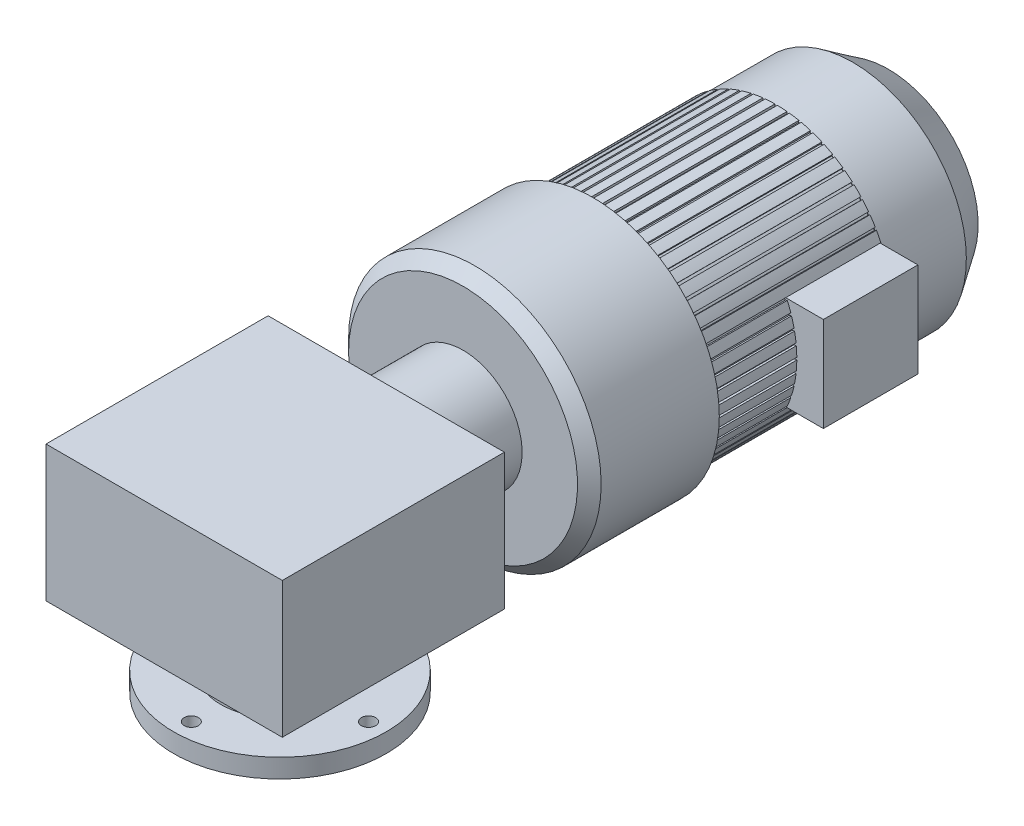
SolidWorks part; units mm, degrees
ref_plane "Front Plane" through (0, 0, 0) normal (0, 0, 1) x (1, 0, 0)
ref_plane "Top Plane" through (0, 0, 0) normal (0, 1, 0) x (1, 0, 0)
ref_plane "Right Plane" through (0, 0, 0) normal (1, 0, 0) x (0, 0, -1)
sketch "Sketch1" plane through (0, 0, 0) normal (0, 0, 1) x (1, 0, 0)
  circle A0 centre (0, 0) radius 16
  dimension "D1" = 32
extrude "Boss-Extrude1" add sketch "Sketch1" along normal blind 55 contours A0
sketch "Sketch2" plane through (0, 0, 0) normal (0, 0, -1) x (-1, 0, 0)
  circle A0 centre (0, 0) radius 22.5
  dimension "D1" = 45
extrude "Boss-Extrude2" add sketch "Sketch2" along normal blind 5
sketch "Sketch3" plane through (0, 0, -5) normal (0, 0, -1) x (-1, 0, 0)
  circle A0 centre (0, 0) radius 25
  dimension "D1" = 50
extrude "Boss-Extrude3" add sketch "Sketch3" along normal blind 5
sketch "Sketch4" plane through (0, 0, -10) normal (0, 0, -1) x (-1, 0, 0)
  circle A0 centre (0, -30.4) radius 50
  dimension "D2" = 100
  dimension "D1" = 30.4
extrude "Boss-Extrude4" add sketch "Sketch4" along normal blind 65
sketch "Sketch5" plane through (0, 0, -75) normal (0, 0, -1) x (-1, 0, 0)
  circle A0 centre (0, -30.4) radius 106.9
  dimension "D1" = 213.8
extrude "Boss-Extrude5" add sketch "Sketch5" along normal blind 110
sketch "Sketch6" plane through (0, 0, -185) normal (0, 0, -1) x (-1, 0, 0)
  circle A0 centre (0, -30.4) radius 97.5
  dimension "D1" = 195
extrude "Boss-Extrude6" add sketch "Sketch6" along normal blind 155
sketch "Sketch7" plane through (0, 0, -340) normal (0, 0, -1) x (-1, 0, 0)
  line L1 (-1, 69.1) -> (1, 69.1)
  line L2 (-1, 69.1) -> (-1, 65.1)
  line L3 (-1, 65.1) -> (1, 65.1)
  line L4 (1, 69.1) -> (1, 65.1)
  line L5 (-1, 69.1) -> (1, 65.1) construction
  line L6 (-1, 65.1) -> (1, 69.1) construction
  circle A0 centre (0, -30.4) radius 97.5 construction
  circle A1 centre (0, -30.4) radius 97.5 construction
  point P0 (0, 67.1)
  dimension "D1" = 2
  dimension "D2" = 2
extrude "Cut-Extrude1" cut sketch "Sketch7" against normal up to surface (155 mm away) up to face at (-97.5, -30.4, -185)
pattern_circular "CirPattern1" count 60 over 360 about axis through (0, -30.4, 0) along (0, 0, 1) of "Cut-Extrude1"
sketch "Sketch8" plane through (0, 0, -340) normal (0, 0, -1) x (-1, 0, 0)
  circle A0 centre (0, -30.4) radius 96
  dimension "D1" = 192
extrude "Boss-Extrude7" add sketch "Sketch8" along normal blind 95
chamfer "Chamfer1" distance 30 distance2 20 1 edges at (-96, -30.4, -435)
sketch "Sketch13" plane through (0, 0, 0) normal (1, 0, 0) x (0, 0, -1)
  line L0 (405, -30.4) -> (75, -30.4) construction
  line L1 (405, -126.4) -> (405, 65.6) construction
  line L2 (75, 76.5) -> (75, -137.3) construction
  line L4 (340, 9.6) -> (260, 9.6)
  line L5 (340, 9.6) -> (340, -70.4)
  line L6 (340, -70.4) -> (260, -70.4)
  line L7 (260, 9.6) -> (260, -70.4)
  line L8 (340, 9.6) -> (260, -70.4) construction
  line L9 (340, -70.4) -> (260, 9.6) construction
  point P6 (300, -30.4)
  dimension "D1" = 80
  dimension "D2" = 80
  dimension "D3" = 105
sketch "Sketch14" plane through (0, 0, -10) normal (0, 0, 1) x (1, 0, 0)
  line L1 (-100, -87.6984) -> (100, -87.6984)
  line L2 (-100, -87.6984) -> (-100, 27.3016)
  line L3 (-100, 27.3016) -> (100, 27.3016)
  line L4 (100, -87.6984) -> (100, 27.3016)
  line L5 (-100, -87.6984) -> (100, 27.3016) construction
  line L6 (-100, 27.3016) -> (100, -87.6984) construction
  circle A0 centre (0, -30.4) radius 50 construction
  point P0 (0, -30.1984)
  dimension "D1" = 200
  dimension "D2" = 100
  dimension "D3" = 115
extrude "Boss-Extrude8" add sketch "Sketch13" along normal blind 120
extrude "Boss-Extrude9" add sketch "Sketch14" along normal blind 188
sketch "Sketch15" plane through (0, -87.6984, 0) normal (0, -1, 0) x (-1, 0, 0)
  line L0 (100, 10) -> (-100, 10) construction
  line L1 (100, -178) -> (100, 10) construction
  circle A0 centre (0, -80) radius 50
  dimension "D1" = 100
  dimension "D2" = 90
  dimension "D3" = 100
extrude "Boss-Extrude10" add sketch "Sketch15" along normal blind 50
sketch "Sketch16" plane through (0, -137.6984, 0) normal (0, -1, 0) x (-1, 0, 0)
  circle A0 centre (0, -80) radius 90
  circle A1 centre (0, -80) radius 75 construction
  circle A2 centre (0, -5) radius 6
  circle A3 centre (-75, -80) radius 6
  circle A4 centre (75, -80) radius 6
  circle A5 centre (0, -155) radius 6
  dimension "D1" = 180
  dimension "D2" = 150
  dimension "D3" = 12
  dimension "D4" = 12
  dimension "D5" = 12
  dimension "D6" = 12
extrude "Boss-Extrude11" add sketch "Sketch16" along normal blind 16
chamfer "Chamfer2" distance 10 angle 45 1 edges at (-106.9, -30.4, -75)
